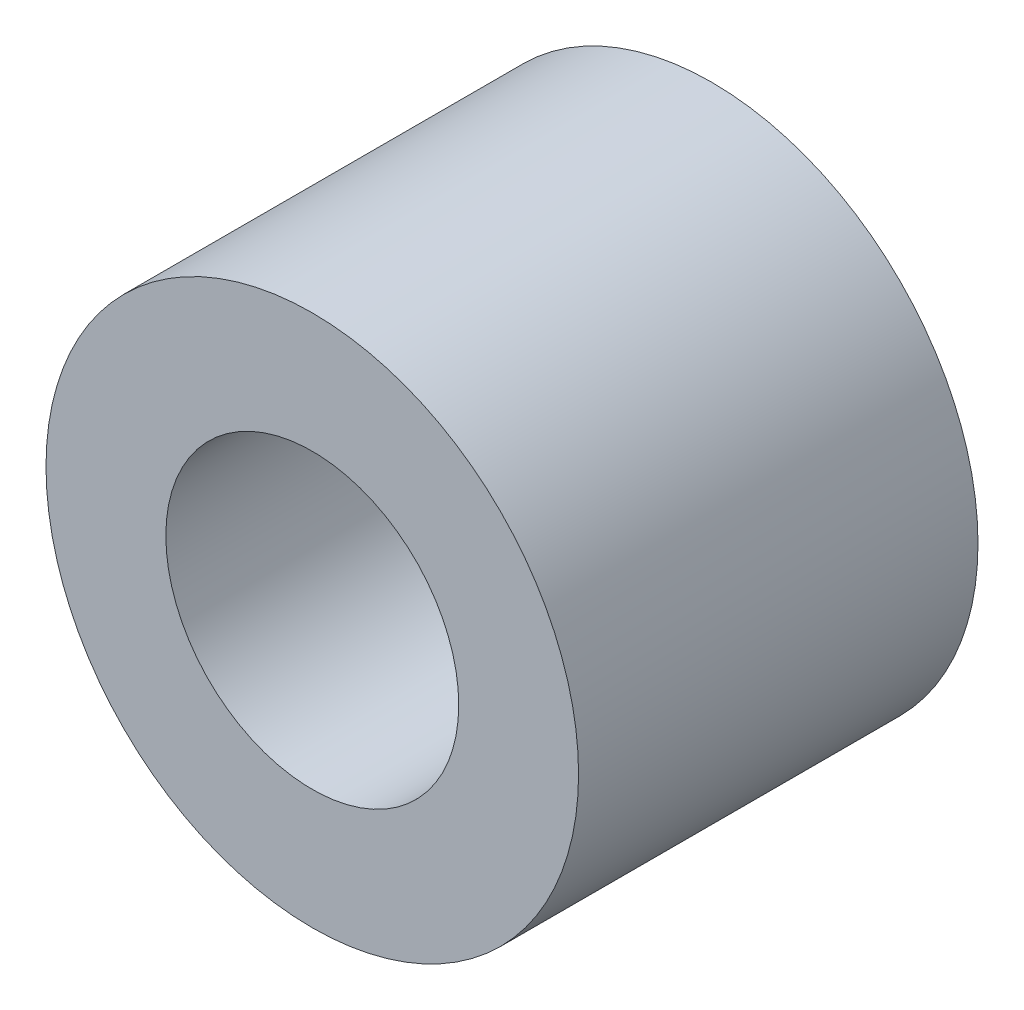
SolidWorks part; units mm, degrees
material "柔性聚氨酯泡沫体"
ref_plane "前视基准面" through (0, 0, 0) normal (0, 0, 1) x (1, 0, 0)
ref_plane "上视基准面" through (0, 0, 0) normal (0, 1, 0) x (1, 0, 0)
ref_plane "右视基准面" through (0, 0, 0) normal (1, 0, 0) x (0, 0, -1)
sketch "草图1" plane through (0, 0, 0) normal (0, 0, 1) x (1, 0, 0)
  circle A0 centre (0, 0) radius 10
  dimension "D1" = 20
extrude "凸台-拉伸1" add sketch "草图1" along normal blind 15
hole_wizard "打孔尺寸(%根据)内六角圆柱头螺钉的类型1" positions "草图2" profile "草图3" counterbore size "M6" standard "GB" end condition through all
sketch "草图2" plane through (0, 0, 15) normal (0, 0, 1) x (1, 0, 0)
  point P0 (0, 0)
sketch "草图3" plane through (0, 0, 15) normal (1, 0, 0) x (0, -1, 0)
  line L0 (0, 0) -> (0, 15)
  line L1 (0, 15) -> (3.3, 15)
  line L3 (3.3, 15) -> (3.3, 8)
  line L4 (3.3, 8) -> (5.5, 8)
  line L5 (5.5, 8) -> (5.5, 0)
  line L7 (5.5, 0) -> (0, 0)
  line L11 (0, -6.35) -> (0, 107.95) construction
  dimension "通孔孔直径" = 6.6
  dimension "通孔孔深度" = 15
  dimension "柱形沉头孔直径" = 11
  dimension "柱形沉头孔深度" = 8
